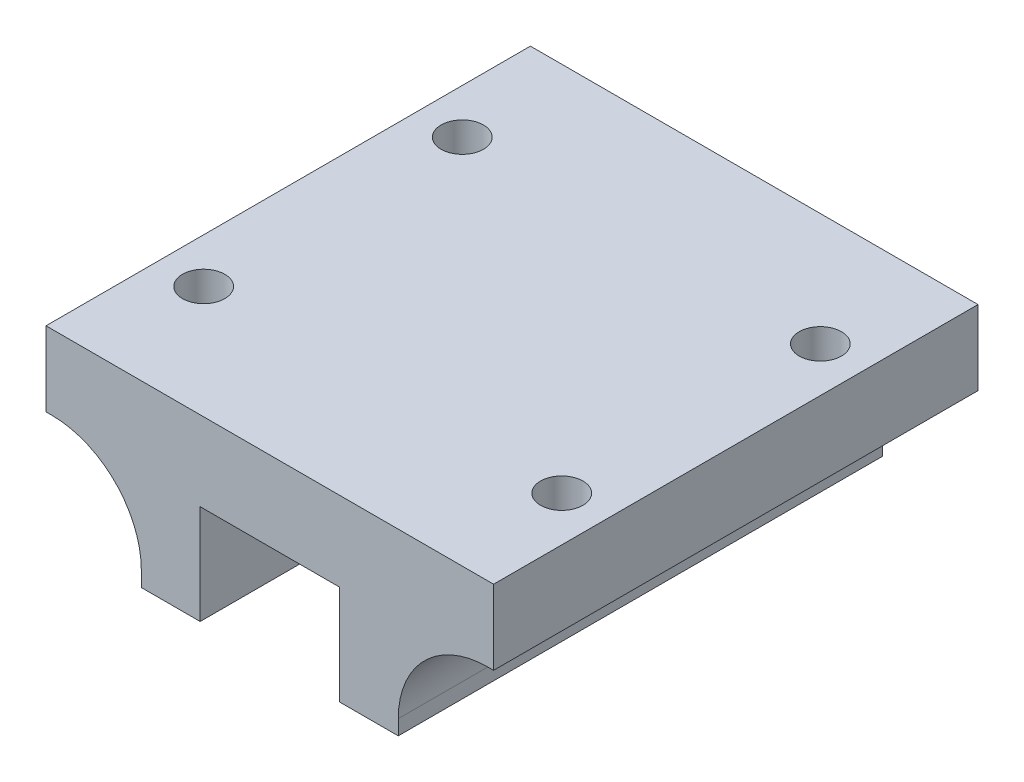
from build123d import *

# Parameters (mm, degrees)
BOSS_EXTRUDE1_DEPTH    = 48.7
M10_TAPPED_HOLE1_D     = 8.5
M10_TAPPED_HOLE1_DEPTH = 24.5
M10_TAPPED_HOLE1_TIP   = 2.553657631


with BuildPart() as part:
    # Sketch1 → Boss-Extrude1 (new, symmetric)
    with BuildSketch(Plane.XY):
        with BuildLine():
            Line((-25.830388506, -36), (-25.830388506, -33))
            ThreePointArc((-25.830388506, -33), (-31.102466444, -20.272077939), (-43.830388506, -15))
            Line((-43.830388506, -15), (-45, -15))
            Line((-45, -15), (-45, 0))
            Line((-45, 0), (45, 0))
            Line((45, 0), (45, -15))
            Line((45, -15), (43.830388506, -15))
            ThreePointArc((43.830388506, -15), (31.102466444, -20.272077939), (25.830388506, -33))
            Line((25.830388506, -33), (25.830388506, -36))
            Line((25.830388506, -36), (14, -36))
            Line((14, -36), (14, -16))
            Line((14, -16), (-14, -16))
            Line((-14, -16), (-14, -36))
            Line((-14, -36), (-25.830388506, -36))
        make_face()
    extrude(amount=BOSS_EXTRUDE1_DEPTH, both=True)

    # M10 Tapped Hole1
    with Locations(Plane(origin=(0, 0, 0), x_dir=(-1, 0, 0), z_dir=(0, 1, 0))):
        with Locations((-36, 26), (36, 26), (-36, -26), (36, -26)):
            Hole(M10_TAPPED_HOLE1_D / 2, depth=M10_TAPPED_HOLE1_DEPTH)
            with Locations((0, 0, -(M10_TAPPED_HOLE1_DEPTH + M10_TAPPED_HOLE1_TIP / 2))):  # 118° drill point
                Cone(0, M10_TAPPED_HOLE1_D / 2, M10_TAPPED_HOLE1_TIP, mode=Mode.SUBTRACT)


solid = part.part
